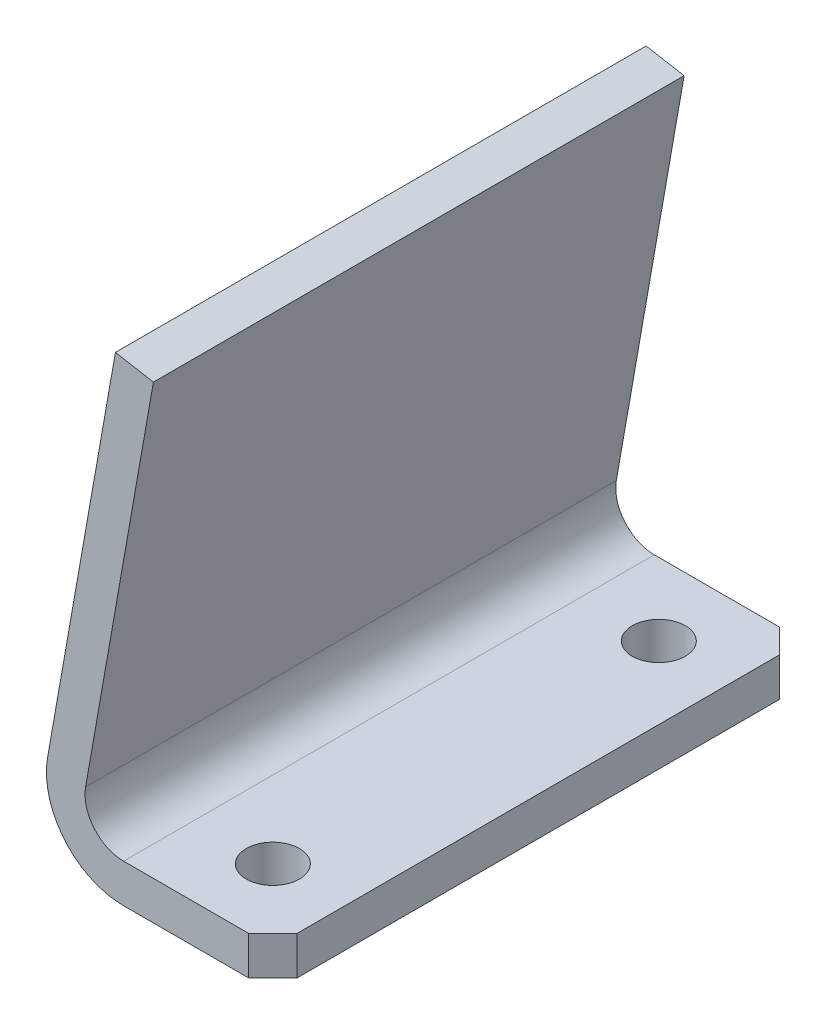
SolidWorks part; units mm, degrees
material "1023 碳钢板 (SS)"
ref_plane "前视基准面" through (0, 0, 0) normal (0, 0, 1) x (1, 0, 0)
ref_plane "上视基准面" through (0, 0, 0) normal (0, 1, 0) x (1, 0, 0)
ref_plane "右视基准面" through (0, 0, 0) normal (1, 0, 0) x (0, 0, -1)
ref_plane "基准面4" through (0, 0, 110) normal (0, 0, 1) x (1, 0, 0)
sketch "草图1" plane through (0, 0, 110) normal (0, 0, 1) x (1, 0, 0)
  line L0 (50, 0) -> (50, 92.7263)
  line L1 (50, 92.7263) -> (17.3648, 98.4808)
  line L2 (17.3648, 98.4808) -> (0, 0)
  line L3 (0, 0) -> (50, 0)
extrude "凸台-拉伸1" add sketch "草图1" against normal blind 110
sketch "草图2" plane through (0, 0, 0) normal (0, 0, -1) x (-1, 0, 0)
  line L0 (-9.534, 8) -> (-25.2433, 97.0916)
  line L1 (-25.2433, 97.0916) -> (-50, 92.7263)
  line L2 (-50, 92.7263) -> (-50, 8)
  line L3 (-50, 8) -> (-9.534, 8)
extrude "切除-拉伸1" cut sketch "草图2" against normal through all
hole_wizard "Ø11.0 (11) 直径孔1" positions "草图4" profile "草图3" hole size "Ø11.0" standard "ANSI Metric"
sketch "草图4" plane through (0, 8, 0) normal (0, 1, 0) x (1, 0, 0)
  point P0 (35, -15)
  point P1 (35, -95)
sketch "草图3" plane through (35, 8, 15) normal (1, 0, 0) x (0, 0, 1)
  line L0 (0, 0) -> (0, 8)
  line L1 (0, 8) -> (5.5, 8)
  line L2 (5.5, 8) -> (5.5, 0)
  line L5 (5.5, 0) -> (0, 0)
  line L11 (0, -6.35) -> (0, 107.95) construction
  dimension "通孔孔直径" = 11
  dimension "通孔孔深度" = 8
chamfer "倒角1" distance 5 angle 45 2 edges at (50, 4, 0) (50, 4, 110)
fillet "圆角1" radius 8 1 edges at (9.534, 8, 55)
fillet "圆角2" radius 16 1 edges at (0, 0, 55)
